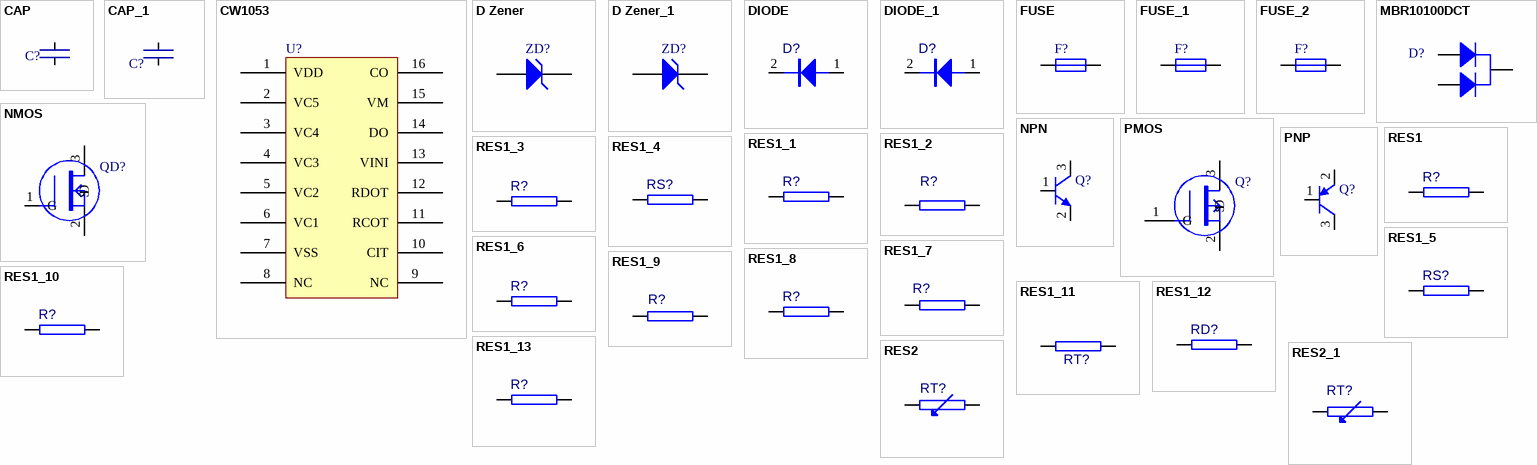
[diagram p0: symbols CAP to RES2_1]
# Altium schematic symbol library MISC86331.SCHLIB: 31 symbols
Pins are listed as number, name and electrical type; pins without a type are passive.


## CAP
designator C?
CAP
footprint C0805A
footprint C0603A (SMD capacitor)
footprint C0603A
footprint C0603A
footprint CAP0805
pins: 1, 2

## CAP_1
designator C?
CAP
footprint CAP0603 (CAP0402)
footprint C0603A (SMD capacitor)
footprint C0603A
pins: 1, 2

## CW1053
designator U?
footprint SO-16
footprint TO-252-A
pins: 1 VDD, 2 VC5, 3 VC4, 4 VC3, 5 VC2, 6 VC1, 7 VSS, 8 NC, 9 NC, 10 CIT, 11 RCOT, 12 RDOT, 13 VINI, 14 DO, 15 VM, 16 CO

## D Zener
designator ZD?
Zener Diode
footprint SOD323
simulation model ZENER (Diode)
signal-integrity model D Zener
pins: 1 A, 2 K

## D Zener_1
designator ZD?
Zener Diode
footprint SOD323
simulation model ZENER (Diode)
signal-integrity model D Zener
pins: 1 A, 2 K

## DIODE
designator D?
DIODE
footprint DIODE0.4
footprint DIODE0.1
footprint DIODE0.3
footprint DIODE0.5
footprint SOD323
pins: 1 A, 2 K
2 alternate drawings of the same symbol

## DIODE_1
designator D?
DIODE
footprint DIODE0.4
footprint DIODE0.1
footprint DIODE0.3
footprint DIODE0.5
footprint SMB-1
footprint SMC
footprint SMB-1
pins: 1 A, 2 K
2 alternate drawings of the same symbol

## FUSE
designator F?
footprint 2410
footprint R1206
pins: 1, 2

## FUSE_1
designator F?
footprint 2410
footprint R1206
pins: 1, 2

## FUSE_2
designator F?
footprint 2410
pins: 1, 2

## MBR10100DCT
designator D?
SMD dual common-cathode diode
footprint TO-252-DIODE-DUAL (SMD diode)
footprint TO-252-A
footprint SMC
pins: 1 A, 2 A, 3 K

## NMOS
designator QD?
footprint SOT-23-3
footprint TO-252
footprint to-252-A
footprint TO-252-A
footprint TO-252-A
pins: 1 G, 2 S, 3 D

## NPN
designator Q?
NPN Bipolar Transistor
footprint TO-226-AA (TO, Flat Index; 3 In-Line, Axial Leads; Body Dia. 4.8mm; Leads 0.55 x 0.51 mm (max))
simulation model NPN
signal-integrity model NPN
footprint SOT-23-3
pins: 1 B, 2, 3 C

## PMOS
designator Q?
footprint SOT-23-3
footprint TO-252-A
footprint SOT-23-3
pins: 1 G, 2 S, 3 D
2 alternate drawings of the same symbol

## PNP
designator Q?
PNP Bipolar Transistor
footprint SOT-23B_N (SOT23, 3-Leads, Body 2.9x1.3mm, Pitch 0.95mm, Lead Span 2.4mm, IPC Medium Density)
footprint SOT-23B_L (SOT23, 3-Leads, Body 2.9x1.3mm, Pitch 0.95mm, Lead Span 2.4mm, IPC High Density)
footprint SOT-23B_M (SOT23, 3-Leads, Body 2.9x1.3mm, Pitch 0.95mm, Lead Span 2.4mm, IPC Low Density)
simulation model PNP
signal-integrity model PNP
footprint SOT-23-3
pins: 1 B, 2 E, 3 C

## RES1
designator R?
RES
footprint AXIAL0.3
footprint AXIAL0.4
footprint AXIAL0.5
footprint AXIAL0.6
footprint 0603
footprint R0603
footprint R0805A
footprint R0805
footprint R0603A (SMD resistor)
footprint RES0805
pins: 1, 2
2 alternate drawings of the same symbol

## RES1_1
designator R?
RES
footprint AXIAL0.3
footprint AXIAL0.4
footprint AXIAL0.5
footprint AXIAL0.6
footprint 0603
footprint R0603
footprint R0603A
footprint RES0603 (CAP0402)
footprint R0603A (SMD resistor)
pins: 1, 2
2 alternate drawings of the same symbol

## RES1_2
designator R?
RES
footprint AXIAL0.3
footprint AXIAL0.4
footprint AXIAL0.5
footprint AXIAL0.6
footprint 0603
footprint R0603
footprint R0603A
footprint RES0603 (CAP0402)
footprint R0603A (SMD resistor)
pins: 1, 2
2 alternate drawings of the same symbol

## RES1_3
designator R?
RES
footprint AXIAL0.3
footprint AXIAL0.4
footprint AXIAL0.5
footprint AXIAL0.6
footprint 0603
footprint R0603
footprint R0603A
footprint RES0603 (CAP0402)
footprint R0603A (SMD resistor)
pins: 1, 2
2 alternate drawings of the same symbol

## RES1_4
designator RS?
RES
footprint AXIAL0.3
footprint AXIAL0.4
footprint AXIAL0.5
footprint AXIAL0.6
footprint 0603
footprint R0603A
footprint 2512
footprint R0603A (SMD resistor)
pins: 1, 2
2 alternate drawings of the same symbol

## RES1_5
designator RS?
RES
footprint AXIAL0.3
footprint AXIAL0.4
footprint AXIAL0.5
footprint AXIAL0.6
footprint 0603
footprint R0603A
footprint 2512
footprint R0603A (SMD resistor)
pins: 1, 2
2 alternate drawings of the same symbol

## RES1_6
designator R?
RES
footprint AXIAL0.3
footprint AXIAL0.4
footprint AXIAL0.5
footprint AXIAL0.6
footprint 0603
footprint R0603A
footprint RES0603 (CAP0402)
footprint R0603A (SMD resistor)
pins: 1, 2
2 alternate drawings of the same symbol

## RES1_7
designator R?
RES
footprint AXIAL0.3
footprint AXIAL0.4
footprint AXIAL0.5
footprint AXIAL0.6
footprint 0603
footprint R0603A
footprint RES0603 (CAP0402)
footprint R0603A (SMD resistor)
pins: 1, 2
2 alternate drawings of the same symbol

## RES1_8
designator R?
RES
footprint AXIAL0.3
footprint AXIAL0.4
footprint AXIAL0.5
footprint AXIAL0.6
footprint 0603
footprint R0603A
footprint RES0603 (CAP0402)
footprint R0603A (SMD resistor)
pins: 1, 2
2 alternate drawings of the same symbol

## RES1_9
designator R?
RES
footprint AXIAL0.3
footprint AXIAL0.4
footprint AXIAL0.5
footprint AXIAL0.6
footprint 0603
footprint R0603
footprint R0603A
footprint RES0603 (CAP0402)
footprint R0603A (SMD resistor)
pins: 1, 2
2 alternate drawings of the same symbol

## RES1_10
designator R?
RES
footprint AXIAL0.3
footprint AXIAL0.4
footprint AXIAL0.5
footprint AXIAL0.6
footprint 0603
footprint R0603A
footprint RES0603 (CAP0402)
footprint R0603A (SMD resistor)
pins: 1, 2
2 alternate drawings of the same symbol

## RES1_11
designator RT?
RES
footprint AXIAL0.3
footprint AXIAL0.4
footprint AXIAL0.5
footprint AXIAL0.6
footprint 0603
footprint R0603
footprint R0603A
footprint RES0603 (CAP0402)
footprint R0603A (SMD resistor)
pins: 1, 2
2 alternate drawings of the same symbol

## RES1_12
designator RD?
RES
footprint AXIAL0.3
footprint AXIAL0.4
footprint AXIAL0.5
footprint AXIAL0.6
footprint 0603
footprint R0603A
footprint RES0603 (CAP0402)
footprint R0603A (SMD resistor)
pins: 1, 2
2 alternate drawings of the same symbol

## RES1_13
designator R?
RES
footprint AXIAL0.3
footprint AXIAL0.4
footprint AXIAL0.5
footprint AXIAL0.6
footprint 0603
footprint RES0603 (CAP0402)
footprint R0603A
footprint RES0603 (CAP0402)
footprint R1206A (SMD resistor)
footprint R0603A (SMD resistor)
footprint R1206
pins: 1, 2
2 alternate drawings of the same symbol

## RES2
designator RT?
RES
footprint SIP-2
footprint WK
footprint R0603A (SMD resistor)
pins: 1, 2
2 alternate drawings of the same symbol

## RES2_1
designator RT?
RES
footprint R0603A
footprint RES0603 (CAP0402)
footprint R0603A (SMD resistor)
pins: 1, 2
2 alternate drawings of the same symbol